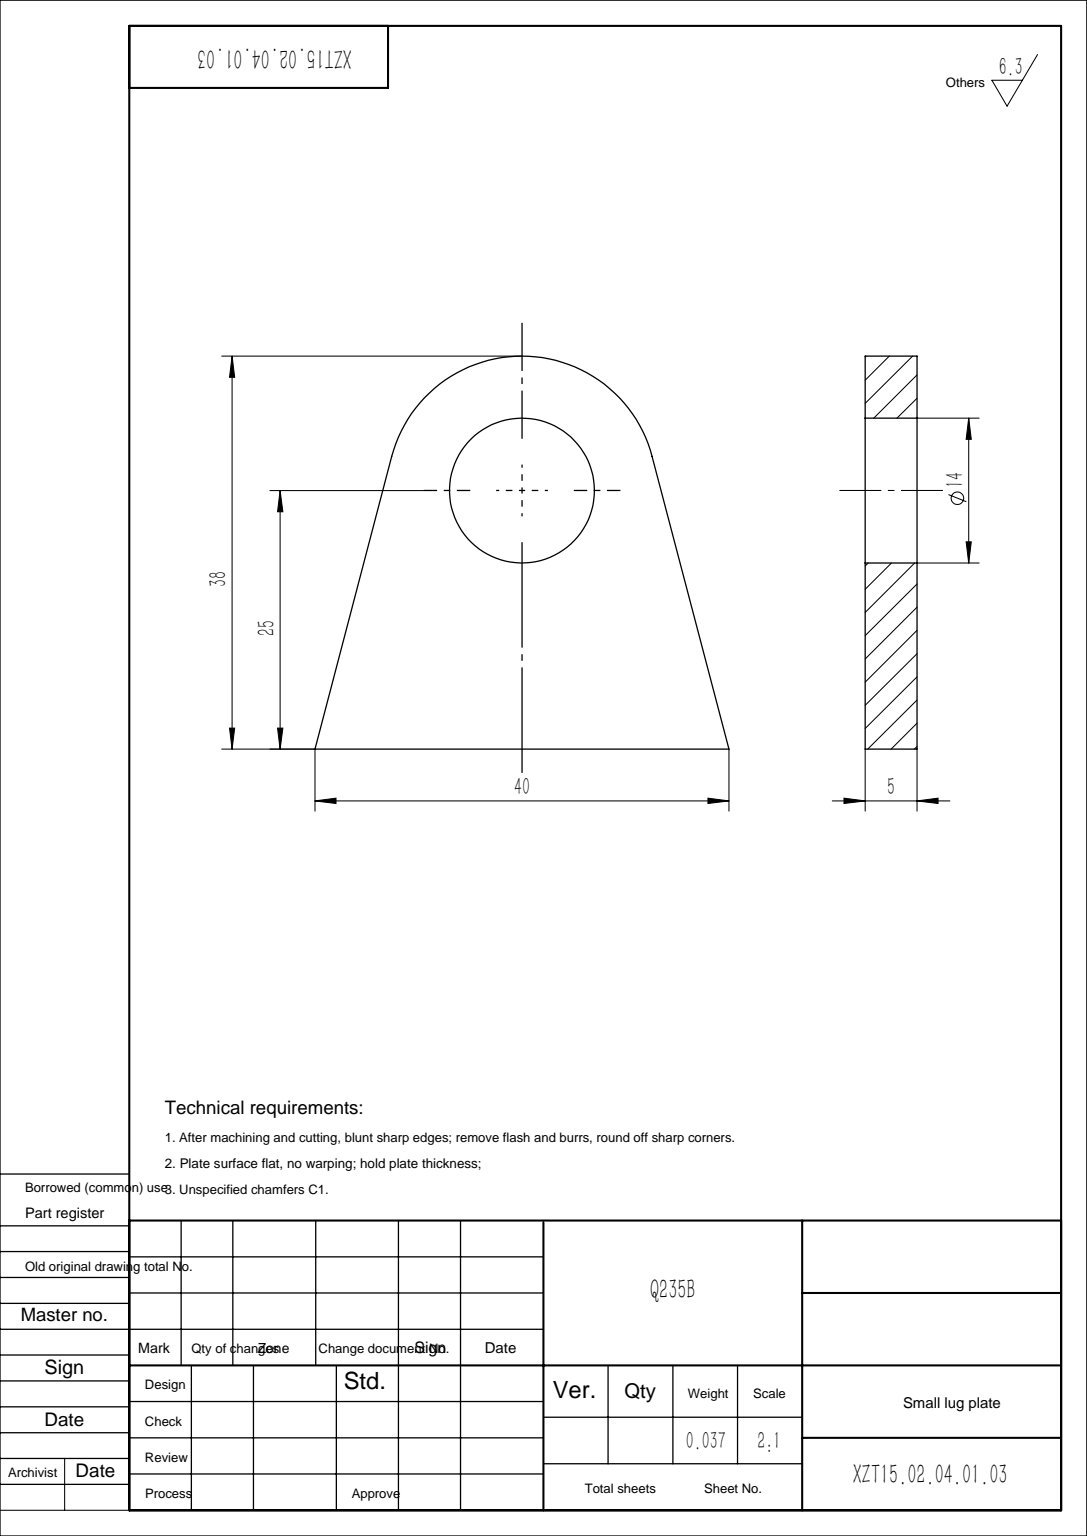
from build123d import *

# Parameters (mm, degrees)
SKETCH1_R           = 7
BOSS_EXTRUDE1_DEPTH = 2.5


with BuildPart() as part:
    # Sketch1 → Boss-Extrude1 (new, symmetric)
    with BuildSketch(Plane.XY):
        with BuildLine():
            Line((20, 0), (-20, 0))
            Line((-20, 0), (-12.57432219, 28.299457752))
            ThreePointArc((-12.57432219, 28.299457752), (0, 38), (12.57432219, 28.299457752))
            Line((12.57432219, 28.299457752), (20, 0))
        make_face()
        with Locations((0, 25)):
            Circle(SKETCH1_R, mode=Mode.SUBTRACT)
    extrude(amount=BOSS_EXTRUDE1_DEPTH, both=True)


solid = part.part
